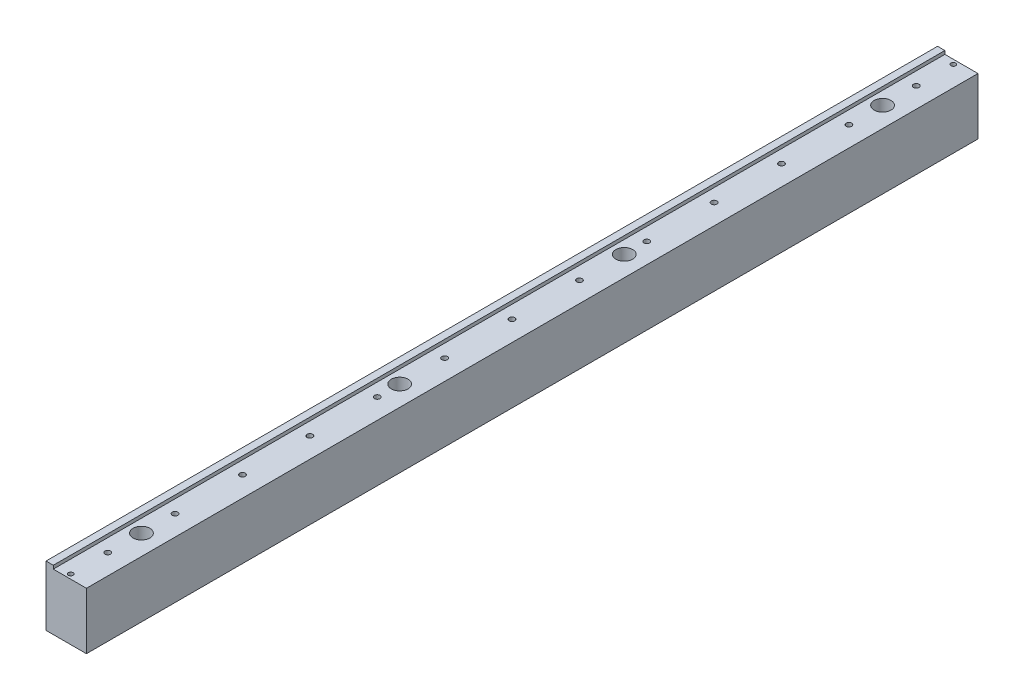
SolidWorks part; units mm, degrees
material "6061 合金"
ref_plane "前视基准面" through (0, 0, 0) normal (0, 0, 1) x (1, 0, 0)
ref_plane "上视基准面" through (0, 0, 0) normal (0, 1, 0) x (1, 0, 0)
ref_plane "右视基准面" through (0, 0, 0) normal (1, 0, 0) x (0, 0, -1)
sketch "草图1" plane through (0, 0, 0) normal (0, 0, 1) x (1, 0, 0)
  line L0 (0, 0) -> (36, 0)
  line L1 (36, 0) -> (36, 50.5)
  line L2 (36, 50.5) -> (6.5, 50.5)
  line L3 (6.5, 50.5) -> (6.5, 53.5)
  line L4 (6.5, 53.5) -> (0, 53.5)
  line L5 (0, 53.5) -> (0, 0)
  dimension "D1" = 36
  dimension "D2" = 6.5
  dimension "D3" = 3
  dimension "D4" = 50.5
extrude "凸台-拉伸1" add sketch "草图1" along normal mid plane 794
hole_wizard "M6 螺纹孔1" positions "草图3" profile "草图2" tap size "M6" standard "GB"
sketch "草图3" plane through (0, 0, 0) normal (-1, 0, 0) x (0, 0, 1)
  line L0 (-397, 53.5) -> (-397, 0) construction
  line L1 (397, 53.5) -> (-397, 53.5) construction
  point P0 (-320, 28.5)
  point P2 (270, 28.5)
  point P5 (-397, 26.75)
  dimension "D1" = 77
  dimension "D2" = 25
  dimension "D3" = 590
sketch "草图2" plane through (0, 28.5, -320) normal (0, 1, 0) x (0, 0, 1)
  line L0 (0, 0) -> (0, 16.5022)
  line L1 (0, 16.5022) -> (2.5, 15)
  line L2 (2.5, 15) -> (2.5, 0)
  line L5 (2.5, 0) -> (0, 0)
  line L10 (0, 16.5022) -> (-2.5, 15) construction
  line L11 (0, -6.35) -> (0, 107.95) construction
  dimension "螺纹孔钻头直径" = 5
  dimension "螺纹孔钻头深度" = 15
  dimension "导头角度" = 118
cosmetic thread "孔螺蚊线2" parameters "D1"=12, "D2"=6
cosmetic thread "孔螺蚊线3" parameters "D1"=12, "D2"=6
hole_wizard "M6 螺纹孔2" positions "草图5" profile "草图4" tap size "M6" standard "GB"
sketch "草图5" plane through (0, 50.5, 0) normal (0, 1, 0) x (1, 0, 0)
  line L0 (6.5, -397) -> (6.5, 397) construction
  line L1 (36, 397) -> (6.5, 397) construction
  point P0 (18, 360)
  dimension "D1" = 11.5
  dimension "D2" = 37
sketch "草图4" plane through (18, 50.5, -360) normal (1, 0, 0) x (0, 0, 1)
  line L0 (0, 0) -> (0, 16.5022)
  line L1 (0, 16.5022) -> (2.5, 15)
  line L2 (2.5, 15) -> (2.5, 0)
  line L5 (2.5, 0) -> (0, 0)
  line L10 (0, 16.5022) -> (-2.5, 15) construction
  line L11 (0, -6.35) -> (0, 107.95) construction
  dimension "螺纹孔钻头直径" = 5
  dimension "螺纹孔钻头深度" = 15
  dimension "导头角度" = 118
cosmetic thread "孔螺蚊线1" parameters "D1"=12, "D2"=6
pattern_linear "阵列(线性)1" count 13 spacing 60 along (0, 0, 1) of "M6 螺纹孔2"
hole_wizard "打孔尺寸(%根据)内六角圆柱头螺钉的类型1" positions "草图7" profile "草图8" counterbore size "M8" standard "GB" end condition through all
sketch "草图7" plane through (0, 50.5, 0) normal (0, 1, 0) x (1, 0, 0)
  line L4 (36, -397) -> (36, 397) construction
  line L6 (0, -397) -> (0, 397) construction
  point P0 (18, 330)
  point P15 (18, 100)
  point P17 (18, -100)
  point P19 (18, -330)
  point P20 (0, 0)
  dimension "D1" = 18
  dimension "D2" = 230
  dimension "D3" = 100
  dimension "D4" = 100
  dimension "D5" = 230
sketch "草图8" plane through (18, 50.5, -330) normal (1, 0, 0) x (0, 0, 1)
  line L0 (0, 0) -> (0, 50.5)
  line L1 (0, 50.5) -> (4.5, 50.5)
  line L3 (4.5, 50.5) -> (4.5, 15)
  line L4 (4.5, 15) -> (7.5, 15)
  line L5 (7.5, 15) -> (7.5, 0)
  line L7 (7.5, 0) -> (0, 0)
  line L11 (0, -6.35) -> (0, 107.95) construction
  dimension "通孔孔直径" = 9
  dimension "通孔孔深度" = 50.5
  dimension "柱形沉头孔直径" = 15
  dimension "柱形沉头孔深度" = 15
hole_wizard "M5 螺纹孔1" positions "草图12" profile "草图11" tap size "M5" standard "GB"
sketch "草图12" plane through (0, 50.5, 0) normal (0, 1, 0) x (1, 0, 0)
  line L0 (36, 397) -> (6.5, 397) construction
  line L1 (0, -397) -> (0, 397) construction
  line L3 (36, -397) -> (6.5, -397) construction
  point P0 (18, 393)
  point P2 (18, -393)
  dimension "D1" = 4
  dimension "D2" = 18
  dimension "D3" = 4
cosmetic thread "孔螺蚊线4" parameters "D1"=10, "D2"=5
cosmetic thread "孔螺蚊线5" parameters "D1"=10, "D2"=5
sketch "草图11" plane through (18, 50.5, -393) normal (1, 0, 0) x (0, 0, 1)
  line L0 (0, 0) -> (0, 13.6618)
  line L1 (0, 13.6618) -> (2.1, 12.4)
  line L2 (2.1, 12.4) -> (2.1, 0)
  line L5 (2.1, 0) -> (0, 0)
  line L10 (0, 13.6618) -> (-2.1, 12.4) construction
  line L11 (0, -6.35) -> (0, 107.95) construction
  dimension "螺纹孔钻头直径" = 4.2
  dimension "螺纹孔钻头深度" = 12.4
  dimension "导头角度" = 118
